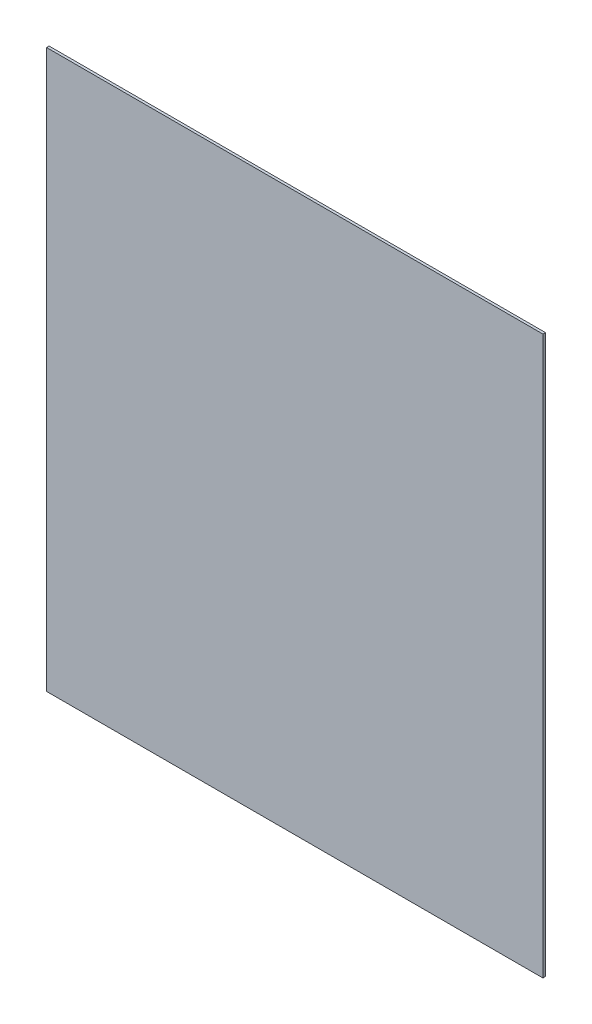
from build123d import *

# Parameters (mm, degrees)
SKETCH_1_W      = 972
SKETCH_1_H      = 1092
EXTRUDE_1_DEPTH = 5


with BuildPart() as part:
    # 草图1 → 凸台-拉伸1 (new body)
    with BuildSketch(Plane.XY):
        Rectangle(SKETCH_1_W, SKETCH_1_H)
    extrude(amount=EXTRUDE_1_DEPTH)


solid = part.part
